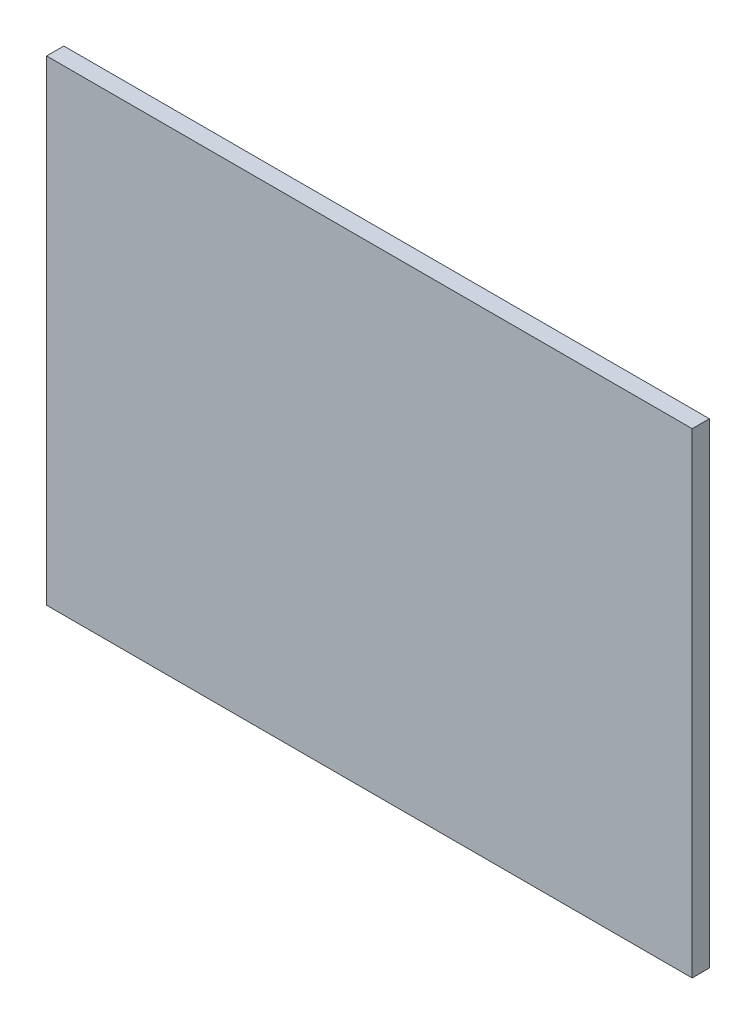
SolidWorks part; units mm, degrees
ref_plane "Front Plane" through (0, 0, 0) normal (0, 0, 1) x (1, 0, 0)
ref_plane "Top Plane" through (0, 0, 0) normal (0, 1, 0) x (1, 0, 0)
ref_plane "Right Plane" through (0, 0, 0) normal (1, 0, 0) x (0, 0, -1)
sketch "Sketch1" plane through (0, 0, 0) normal (0, 0, 1) x (1, 0, 0)
  line L1 (-5.625, -4.145) -> (5.625, -4.145)
  line L2 (-5.625, -4.145) -> (-5.625, 4.145)
  line L3 (-5.625, 4.145) -> (5.625, 4.145)
  line L4 (5.625, -4.145) -> (5.625, 4.145)
  line L5 (-5.625, -4.145) -> (5.625, 4.145) construction
  line L6 (-5.625, 4.145) -> (5.625, -4.145) construction
  point P0 (0, 0)
  dimension "D1" = 11.25
  dimension "D2" = 8.29
extrude "Boss-Extrude1" add sketch "Sketch1" along normal mid plane 0.3
